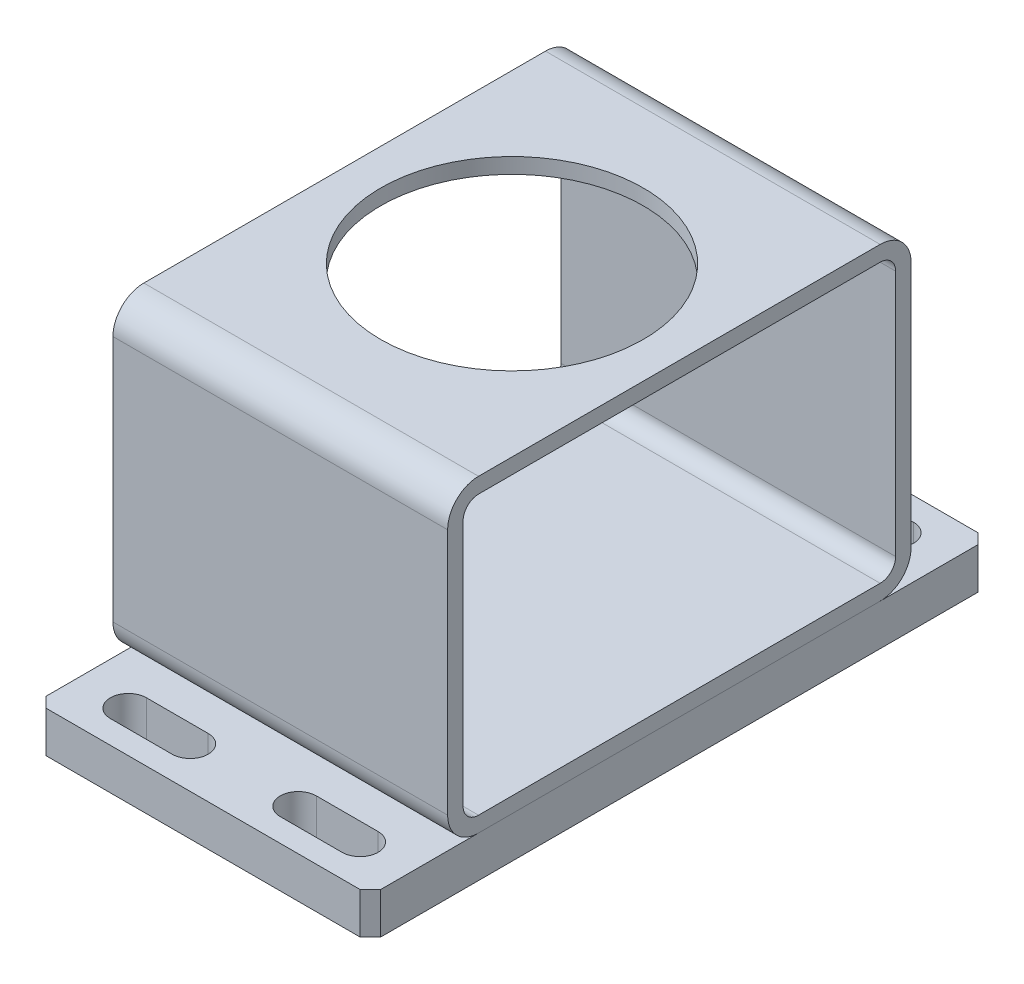
SolidWorks part; units mm, degrees
material "Q235A"
ref_plane "前视基准面" through (0, 0, 0) normal (0, 0, 1) x (1, 0, 0)
ref_plane "上视基准面" through (0, 0, 0) normal (0, 1, 0) x (1, 0, 0)
ref_plane "右视基准面" through (0, 0, 0) normal (1, 0, 0) x (0, 0, -1)
sketch "草图1" plane through (0, 0, 0) normal (0, 0, 1) x (1, 0, 0)
  line L0 (-32.5, 0) -> (32.5, 0)
  point P4 (0, 0)
  dimension "D1" = 65
other "冷弯空心矩管gb∕t6728-2002 90 X 60 X 3(1)"
ref_plane "基准面1" through (-32.5, 0, 0) normal (1, 0, 0) x (0, 1, 0)
sketch "Sketch11" plane through (-32.5, 0, 0) normal (1, 0, 0) x (0, 1, 0)
  line L0 (-24, -42) -> (24, -42)
  line L1 (-27, -39) -> (-27, 39)
  line L2 (24, 42) -> (-24, 42)
  line L3 (27, 39) -> (27, -39)
  line L4 (-24, -45) -> (24, -45)
  line L5 (-30, -39) -> (-30, 39)
  line L6 (24, 45) -> (-24, 45)
  line L7 (30, 39) -> (30, -39)
  arc A0 (30, 39) -> (24, 45) centre (24, 39) ccw
  arc A1 (24, -45) -> (30, -39) centre (24, -39) ccw
  arc A2 (-30, -39) -> (-24, -45) centre (-24, -39) ccw
  arc A3 (-24, 45) -> (-30, 39) centre (-24, 39) ccw
  arc A4 (-24, 42) -> (-27, 39) centre (-24, 39) ccw
  arc A5 (27, 39) -> (24, 42) centre (24, 39) ccw
  arc A6 (24, -42) -> (27, -39) centre (24, -39) ccw
  arc A7 (-27, -39) -> (-24, -42) centre (-24, -39) ccw
  point P0 (0, 45)
  point P1 (30, 0)
  point P2 (0, -45)
  point P3 (-30, 0)
  point P4 (-30, 45)
  point P5 (30, 45)
  point P6 (30, -45)
  point P7 (-30, -45)
  point P8 (0, 0)
  point P33 (0, 0)
  dimension "D1" = 6
  dimension "Thickness" = 3
  dimension "V_leg" = 90
  dimension "H_leg" = 60
sketch "草图4" plane through (0, 30, 0) normal (0, 1, 0) x (1, 0, 0)
  circle A0 centre (0, 0) radius 25.5
  dimension "D1" = 51
extrude "切除-拉伸1" cut sketch "草图4" against normal up to next
sketch "草图5" plane through (0, -30, 0) normal (0, -1, 0) x (1, 0, 0)
  line L0 (32.5, 39) -> (32.5, -39) construction
  line L1 (-32.5, -27.5) -> (32.5, -27.5)
  line L2 (-32.5, -27.5) -> (-32.5, 27.5)
  line L3 (-32.5, 27.5) -> (32.5, 27.5)
  line L4 (32.5, -27.5) -> (32.5, 27.5)
  line L5 (-32.5, -27.5) -> (32.5, 27.5) construction
  line L6 (-32.5, 27.5) -> (32.5, -27.5) construction
  point P0 (0, 0)
  dimension "D1" = 55
extrude "切除-拉伸3" [suppressed] cut sketch "草图5" against normal up to next
sketch "草图6" [suppressed] plane through (0, -30, 0) normal (0, -1, 0) x (1, 0, 0)
  line L0 (-40, 39.5) -> (-28, 39.5) construction
  line L1 (-40, 43) -> (-28, 43)
  line L2 (-40, 36) -> (-28, 36)
  line L3 (50, 27.5) -> (-50, 27.5) construction
  line L4 (-50, 52) -> (-50, 27.5) construction
  line L5 (0, 27.5) -> (0, 52) construction
  line L6 (50, 52) -> (-50, 52) construction
  line L7 (40, 39.5) -> (28, 39.5) construction
  line L8 (40, 43) -> (28, 43)
  line L9 (40, 36) -> (28, 36)
  arc A0 (-40, 43) -> (-40, 36) centre (-40, 39.5) ccw
  arc A1 (-28, 36) -> (-28, 43) centre (-28, 39.5) ccw
  arc A2 (40, 43) -> (40, 36) centre (40, 39.5) cw
  arc A3 (28, 36) -> (28, 43) centre (28, 39.5) cw
  point P2 (-34, 39.5)
  point P17 (34, 39.5)
  dimension "D1" = 3.5
  dimension "D2" = 12
  dimension "D3" = 12
  dimension "D4" = 10
extrude "切除-拉伸4" [suppressed] cut sketch "草图6" against normal up to next
mirror "镜向1" [suppressed] about plane through (0, 0, 0) normal (0, 0, 1)
sketch "草图7" plane through (0, -30, 0) normal (0, -1, 0) x (1, 0, 0)
  line L0 (32.5, 39) -> (32.5, -39) construction
  line L1 (-32.5, -60) -> (32.5, -60)
  line L2 (-32.5, -60) -> (-32.5, 60)
  line L3 (-32.5, 60) -> (32.5, 60)
  line L4 (32.5, -60) -> (32.5, 60)
  line L5 (-32.5, -60) -> (32.5, 60) construction
  line L6 (-32.5, 60) -> (32.5, -60) construction
  point P0 (0, 0)
  dimension "D1" = 120
extrude "凸台-拉伸1" add sketch "草图7" along normal blind 8 separate body
sketch "草图8" plane through (0, -38, 0) normal (0, -1, 0) x (1, 0, 0)
  line L0 (-22.5, 52) -> (-10.5, 52) construction
  line L1 (-22.5, 55.5) -> (-10.5, 55.5)
  line L2 (-22.5, 48.5) -> (-10.5, 48.5)
  line L3 (-32.5, 60) -> (-32.5, -60) construction
  line L4 (-32.5, 0) -> (32.5, 0) construction
  arc A0 (-22.5, 55.5) -> (-22.5, 48.5) centre (-22.5, 52) ccw
  arc A1 (-10.5, 48.5) -> (-10.5, 55.5) centre (-10.5, 52) ccw
  point P2 (-16.5, 52)
  dimension "D1" = 3.5
  dimension "D2" = 12
  dimension "D3" = 10
  dimension "D4" = 52
extrude "切除-拉伸5" cut sketch "草图8" against normal up to surface (11 mm away) up to face at (0, -27, 0)
mirror "镜向2" about plane through (0, 0, 0) normal (1, 0, 0) of "切除-拉伸5"
mirror "镜向3" about plane through (0, 0, 0) normal (0, 0, 1) of "镜向2", "切除-拉伸5"
chamfer "倒角1" distance 2 angle 45 4 edges at (32.5, -34, -60) (-32.5, -34, -60) (32.5, -34, 60) (-32.5, -34, 60)
